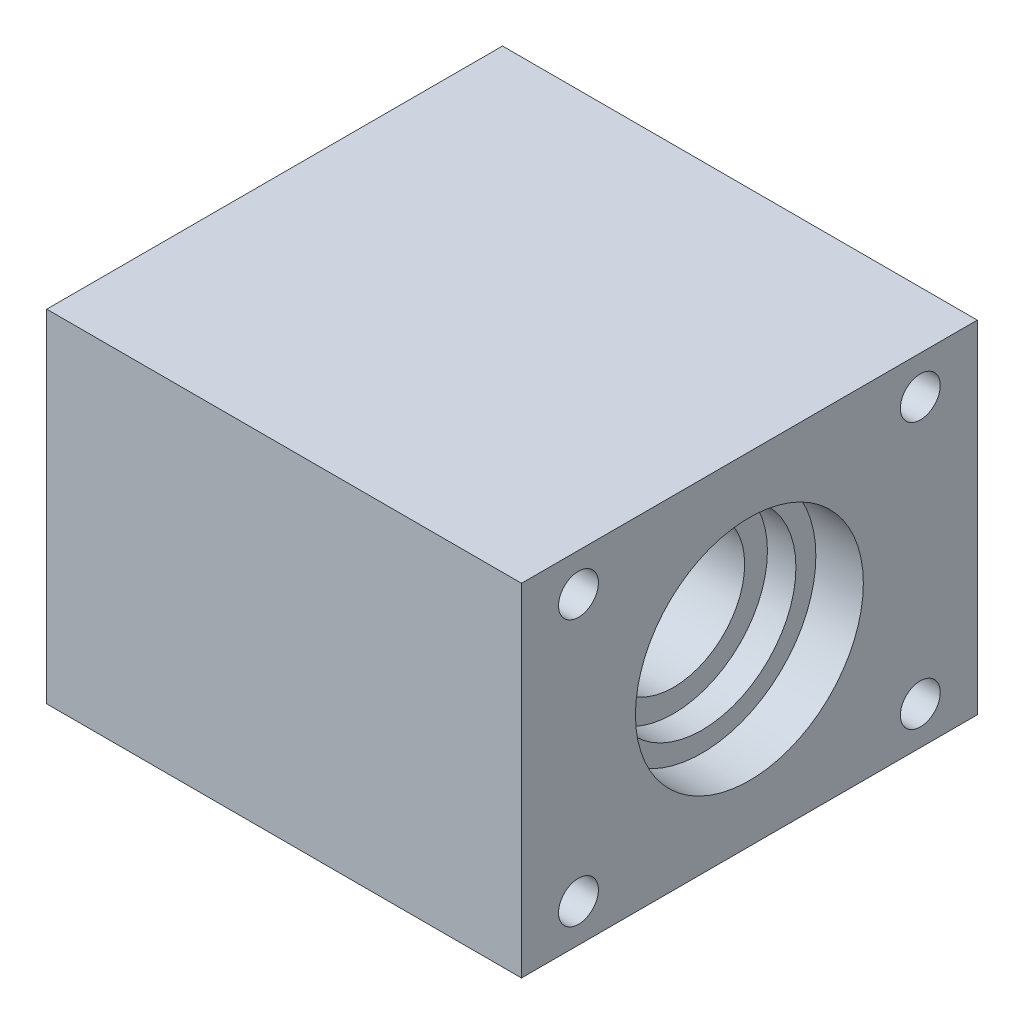
from build123d import *

# Parameters (mm, degrees)
SKETCH1_W             = 48
SKETCH1_H             = 36
SKETCH1_R             = 7.5
BOSS_EXTRUDE1_DEPTH   = 25
SKETCH2_R             = 12
CUT_EXTRUDE1_DEPTH    = 5
SKETCH3_R             = 9.9
CUT_EXTRUDE2_DEPTH    = 3
SKETCH5_R             = 2
CUT_EXTRUDE3_DEPTH    = 20
M5_TAPPED_HOLE1_D     = 4.2
M5_TAPPED_HOLE1_DEPTH = 12.4
M5_TAPPED_HOLE1_TIP   = 1.2618073
M3_TAPPED_HOLE1_D     = 2.5
M3_TAPPED_HOLE1_DEPTH = 10.1
M3_TAPPED_HOLE1_TIP   = 0.751075774


with BuildPart() as part:
    # Sketch1 → Boss-Extrude1 (new, symmetric)
    with BuildSketch(Plane(origin=(0, 0, 0), x_dir=(0, 0, -1), z_dir=(1, 0, 0))):
        Rectangle(SKETCH1_W, SKETCH1_H)
        Circle(SKETCH1_R, mode=Mode.SUBTRACT)
    extrude(amount=BOSS_EXTRUDE1_DEPTH, both=True)

    # Sketch2 → Cut-Extrude1 (cut)
    with BuildSketch(Plane.ZY.offset(25)):
        Circle(SKETCH2_R)
    cut_extrude1 = extrude(amount=-CUT_EXTRUDE1_DEPTH, mode=Mode.SUBTRACT)

    # Sketch3 → Cut-Extrude2 (cut)
    with BuildSketch(Plane.ZY.offset(20)):
        Circle(SKETCH3_R)
    cut_extrude2 = extrude(amount=-CUT_EXTRUDE2_DEPTH, mode=Mode.SUBTRACT)

    # Mirror4: Cut-Extrude1, Cut-Extrude2 across plane
    add(cut_extrude1.mirror(Plane(origin=(0, 0, 0), x_dir=(0, 0, 1), z_dir=(1, 0, 0))), mode=Mode.SUBTRACT)
    add(cut_extrude2.mirror(Plane(origin=(0, 0, 0), x_dir=(0, 0, 1), z_dir=(1, 0, 0))), mode=Mode.SUBTRACT)

    # Sketch5 → Cut-Extrude3 (cut)
    with BuildSketch(Plane(origin=(0, 0, -24), x_dir=(-1, 0, 0), z_dir=(0, 0, -1))):
        with Locations((7, 0)):
            Circle(SKETCH5_R)
        with Locations((-7, 0)):
            Circle(SKETCH5_R)
    extrude(amount=-CUT_EXTRUDE3_DEPTH, mode=Mode.SUBTRACT)

    # M5 Tapped Hole1
    with Locations(Plane(origin=(25, 0, 0), x_dir=(0, 0, -1), z_dir=(1, 0, 0))):
        with Locations((-18, 14), (18, 14), (-18, -14), (18, -14)):
            Hole(M5_TAPPED_HOLE1_D / 2, depth=M5_TAPPED_HOLE1_DEPTH)
            with Locations((0, 0, -(M5_TAPPED_HOLE1_DEPTH + M5_TAPPED_HOLE1_TIP / 2))):  # 118° drill point
                Cone(0, M5_TAPPED_HOLE1_D / 2, M5_TAPPED_HOLE1_TIP, mode=Mode.SUBTRACT)

    # M3 Tapped Hole1
    with Locations(Plane.ZY.offset(25)):
        with Locations((-14, 14), (-14, -14), (14, 14), (14, -14)):
            Hole(M3_TAPPED_HOLE1_D / 2, depth=M3_TAPPED_HOLE1_DEPTH)
            with Locations((0, 0, -(M3_TAPPED_HOLE1_DEPTH + M3_TAPPED_HOLE1_TIP / 2))):  # 118° drill point
                Cone(0, M3_TAPPED_HOLE1_D / 2, M3_TAPPED_HOLE1_TIP, mode=Mode.SUBTRACT)


solid = part.part
